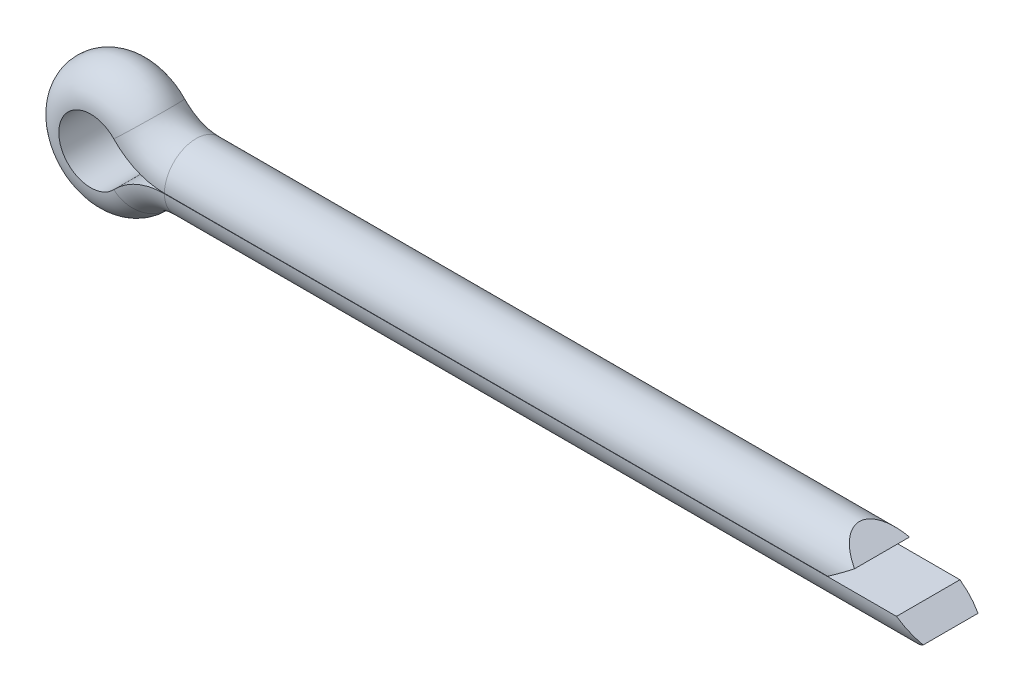
from build123d import *

# Parameters (mm, degrees)
CUT_EXTRUDE_1_DEPTH      = 49.47682334
CUT_EXTRUDE_1_DEPTH_BACK = 49.47682334


with BuildPart() as part:
    # 扫描2: sweep along a path in Sketch 203
    with BuildLine(Plane.XY) as sweep_2_path:
        Line((44.3, 1.85), (4.3, 1.85))
        ThreePointArc((4.3, 1.85), (3.421730256, 2.030913567), (2.686457501, 2.544198517))
        ThreePointArc((2.686457501, 2.544198517), (-3.7, 0), (2.686457501, -2.544198517))
        ThreePointArc((2.686457501, -2.544198517), (3.421730256, -2.030913567), (4.3, -1.85))
        Line((4.3, -1.85), (48.3, -1.85))
    # 草图2 → 扫描2 (sweep)
    with BuildSketch(Plane(origin=(44.3, 1.85, 0), x_dir=(0, 0, 1), z_dir=(-1, 0, 0))):
        with BuildLine():
            Line((-1.849972973, -1.84), (1.849972973, -1.84))
            ThreePointArc((1.849972973, -1.84), (0, 0), (-1.849972973, -1.84))
        make_face()
    sweep(path=sweep_2_path.line)

    # 草图3 → 切除-拉伸1 (cut, two sides: drawn at the far end of the back side and taken through both)
    with BuildSketch(Plane.XY.offset(-CUT_EXTRUDE_1_DEPTH_BACK)):
        Polygon((44.3, 0.92), (42.982464131, 1.85), (48.31, 1.85), (48.31, -1.85), (46.975462056, -1.85), (48.3, -0.93), (46.982464131, 0), (42.975462056, 0), align=None)
    extrude(amount=CUT_EXTRUDE_1_DEPTH + CUT_EXTRUDE_1_DEPTH_BACK, mode=Mode.SUBTRACT)


solid = part.part
